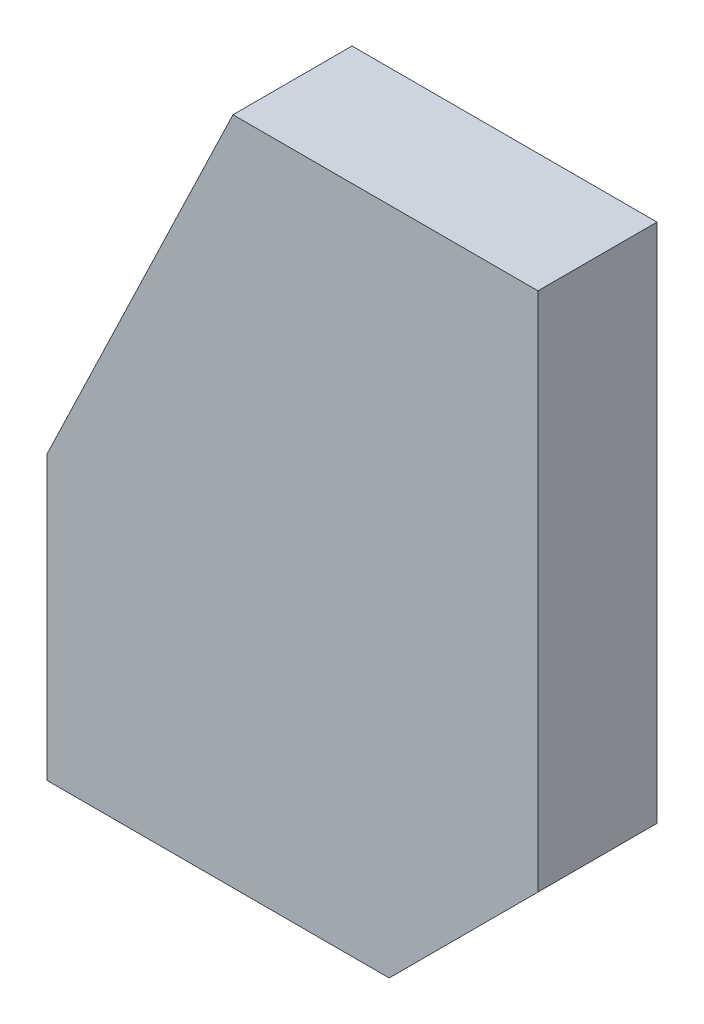
SolidWorks part; units mm, degrees
material "Q235B"
ref_plane "前视基准面" through (0, 0, 0) normal (0, 0, 1) x (1, 0, 0)
ref_plane "上视基准面" through (0, 0, 0) normal (0, 1, 0) x (1, 0, 0)
ref_plane "右视基准面" through (0, 0, 0) normal (1, 0, 0) x (0, 0, -1)
sketch "草图2" plane through (0, 0, 0) normal (0, 0, 1) x (1, 0, 0)
  line L1 (25, 90) -> (66, 90)
  line L2 (66, 90) -> (66, 0)
  line L3 (66, 0) -> (0, 0)
  line L4 (0, 0) -> (0, 38)
  line L5 (0, 38) -> (25, 90)
  dimension "D1" = 66
  dimension "D2" = 90
  dimension "D3" = 41
  dimension "D4" = 38
extrude "凸台-拉伸1" add sketch "草图2" along normal mid plane 16
chamfer "倒角1" distance 20 angle 45 1 edges at (66, 0, 0)
